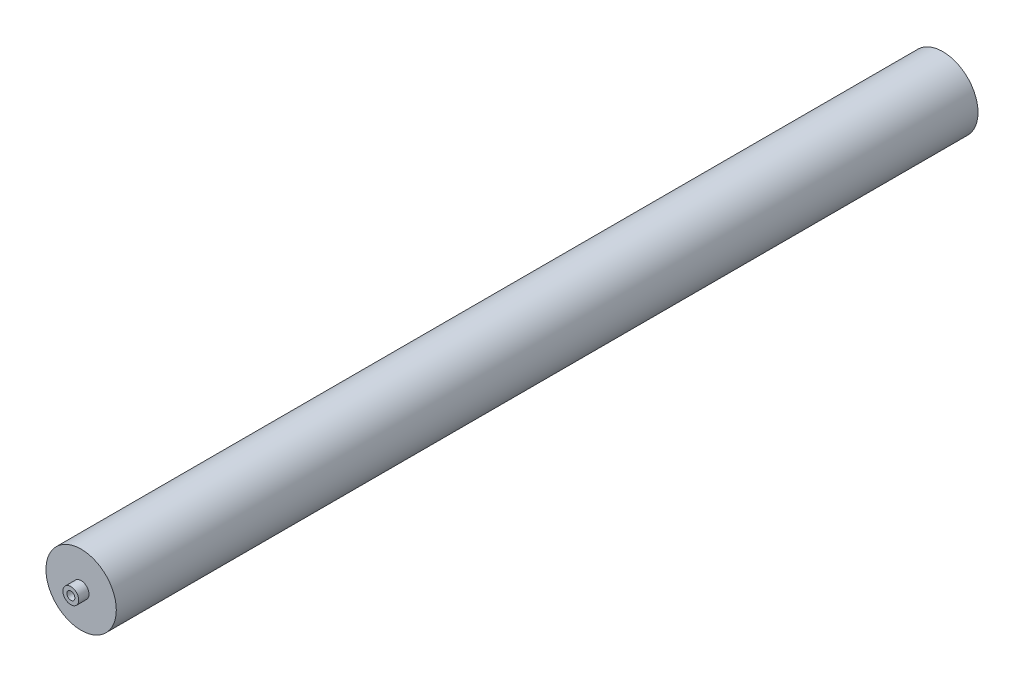
SolidWorks part; units mm, degrees
material "1023 碳钢板 (SS)"
ref_plane "Front Plane" through (0, 0, 0) normal (0, 0, 1) x (1, 0, 0)
ref_plane "Top Plane" through (0, 0, 0) normal (0, 1, 0) x (1, 0, 0)
ref_plane "Right Plane" through (0, 0, 0) normal (1, 0, 0) x (0, 0, -1)
sketch "Sketch1" plane through (0, 0, 0) normal (0, 0, 1) x (1, 0, 0)
  circle A0 centre (0, 0) radius 44.5
  dimension "D1" = 89
extrude "Boss-Extrude1" add sketch "Sketch1" along normal blind 1090
sketch "Sketch2" plane through (0, 0, 1090) normal (0, 0, 1) x (1, 0, 0)
  circle A0 centre (0, 0) radius 10
  dimension "D1" = 20
extrude "Boss-Extrude2" add sketch "Sketch2" along normal blind 13
sketch "Sketch3" plane through (0, 0, 0) normal (0, 0, -1) x (-1, 0, 0)
  circle A0 centre (0, 0) radius 10
  dimension "D1" = 20
extrude "Boss-Extrude3" add sketch "Sketch3" along normal blind 13 contours A0
hole_wizard "M12 Tapped Hole1" positions "Sketch4" profile "Sketch5" tap size "M12" standard "ISO"
sketch "Sketch4" plane through (0, 0, -13) normal (0, 0, -1) x (-1, 0, 0)
  point P0 (0, 0)
sketch "Sketch5" plane through (0, 0, -13) normal (1, 0, 0) x (0, 1, 0)
  line L0 (0, 0) -> (0, 28.3144)
  line L1 (0, 28.3144) -> (5.1, 25.25)
  line L2 (5.1, 25.25) -> (5.1, 0)
  line L5 (5.1, 0) -> (0, 0)
  line L10 (0, 28.3144) -> (-5.1, 25.25) construction
  line L11 (0, -6.35) -> (0, 107.95) construction
  dimension "螺纹孔钻头直径" = 10.2
  dimension "螺纹孔钻头深度" = 25.25
  dimension "导头角度" = 118
cosmetic thread "Hole Thread Line1" parameters "D1"=20, "D2"=12
hole_wizard "M12 Tapped Hole2" positions "Sketch6" profile "Sketch7" tap size "M12" standard "ISO"
sketch "Sketch6" plane through (0, 0, 1103) normal (0, 0, 1) x (1, 0, 0)
  point P0 (0, 0)
sketch "Sketch7" plane through (0, 0, 1103) normal (1, 0, 0) x (0, -1, 0)
  line L0 (0, 0) -> (0, 28.3144)
  line L1 (0, 28.3144) -> (5.1, 25.25)
  line L2 (5.1, 25.25) -> (5.1, 0)
  line L5 (5.1, 0) -> (0, 0)
  line L10 (0, 28.3144) -> (-5.1, 25.25) construction
  line L11 (0, -6.35) -> (0, 107.95) construction
  dimension "螺纹孔钻头直径" = 10.2
  dimension "螺纹孔钻头深度" = 25.25
  dimension "导头角度" = 118
cosmetic thread "Hole Thread Line2" parameters "D1"=20, "D2"=12
